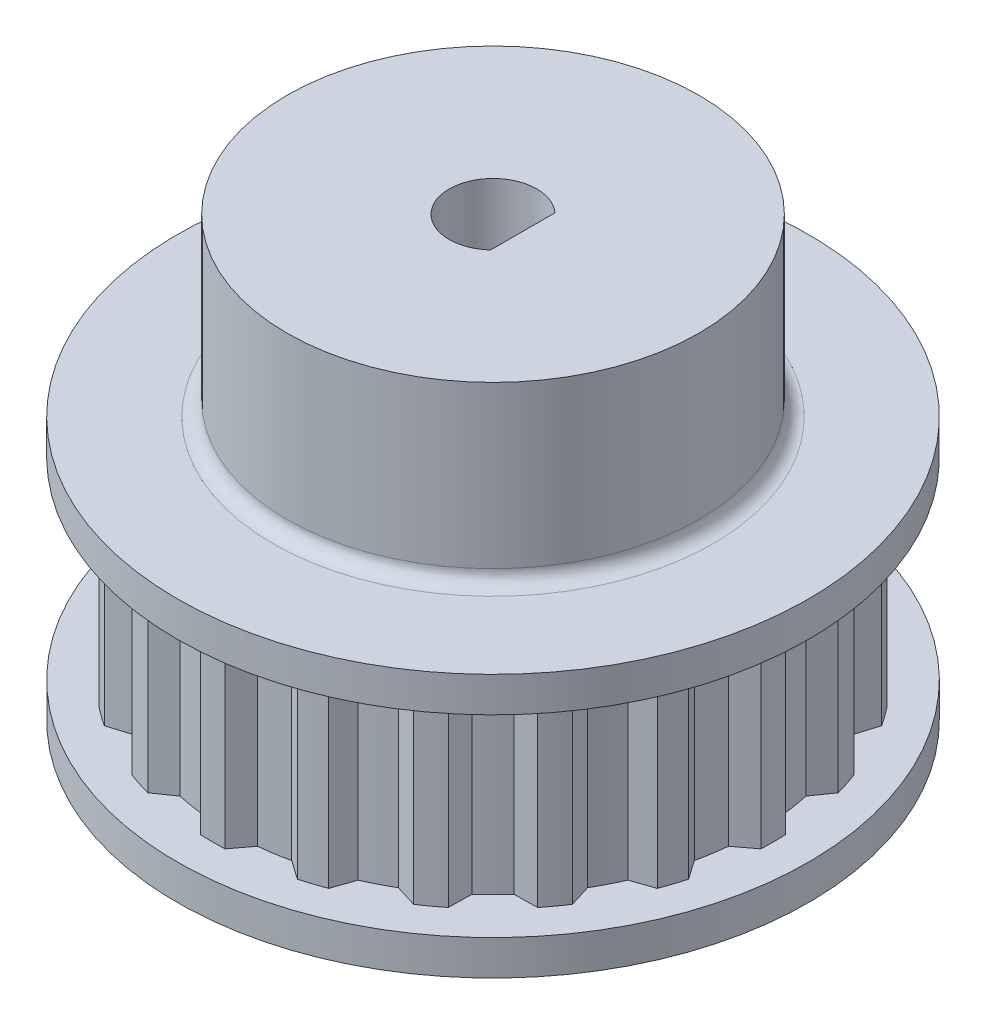
from build123d import *

# Parameters (mm, degrees)
SKETCH1_R           = 16
BOSS_EXTRUDE1_DEPTH = 11
CUT_EXTRUDE2_START  = -21
CUT_EXTRUDE2_DEPTH  = 21
SKETCH3_R           = 18
BOSS_EXTRUDE2_DEPTH = 2
BOSS_EXTRUDE3_START = 2
SKETCH4_R           = 18
BOSS_EXTRUDE3_DEPTH = 2
SKETCH5_R           = 11.75
BOSS_EXTRUDE4_DEPTH = 10
FILLET1_R           = 0.8
CUT_EXTRUDE3_DEPTH  = 52


with BuildPart() as part:
    # Sketch1 → Boss-Extrude1 (new body)
    with BuildSketch(Plane(origin=(0, 0, 0), x_dir=(1, 0, 0), z_dir=(0, 1, 0))):
        with Locations(Location((0, 0, 0), (0, 0, 270))):
            Circle(SKETCH1_R)
    extrude(amount=BOSS_EXTRUDE1_DEPTH)

    # Sketch2 → Cut-Extrude2 (cut)
    with BuildSketch(Plane(origin=(0, 11, 0), x_dir=(1, 0, 0), z_dir=(0, 1, 0)).offset(CUT_EXTRUDE2_START)):
        with BuildLine():
            ThreePointArc((4.265167024, 15.421035966), (2.502951441, 15.80301345), (0.708947293, 15.984285838))
            Line((0.708947293, 15.984285838), (1.5, 14.932939883))
            ThreePointArc((1.5, 14.932939883), (2.347782156, 14.823313142), (3.187947426, 14.665595275))
            Line((3.187947426, 14.665595275), (4.265167024, 15.421035966))
        make_face()
        with BuildLine():
            ThreePointArc((8.821777076, 13.348267649), (7.263847996, 14.256104387), (5.613664909, 14.982882443))
            Line((5.613664909, 14.982882443), (6.041116974, 13.738544292))
            ThreePointArc((6.041116974, 13.738544292), (6.813529192, 13.372303972), (7.563836345, 12.96268002))
            Line((7.563836345, 12.96268002), (8.821777076, 13.348267649))
        make_face()
        with BuildLine():
            ThreePointArc((12.514850122, 9.968877892), (11.313708499, 11.313708499), (9.968877892, 12.514850122))
            Line((9.968877892, 12.514850122), (9.990887328, 11.199324263))
            ThreePointArc((9.990887328, 11.199324263), (10.612320518, 10.612320518), (11.199324263, 9.990887328))
            Line((11.199324263, 9.990887328), (12.514850122, 9.968877892))
        make_face()
        with BuildLine():
            ThreePointArc((14.982882443, 5.613664909), (14.256104387, 7.263847996), (13.348267649, 8.821777076))
            Line((13.348267649, 8.821777076), (12.96268002, 7.563836345))
            ThreePointArc((12.96268002, 7.563836345), (13.372303972, 6.813529192), (13.738544292, 6.041116974))
            Line((13.738544292, 6.041116974), (14.982882443, 5.613664909))
        make_face()
        with BuildLine():
            ThreePointArc((15.984285838, 0.708947293), (15.80301345, 2.502951441), (15.421035966, 4.265167024))
            Line((15.421035966, 4.265167024), (14.665595275, 3.187947426))
            ThreePointArc((14.665595275, 3.187947426), (14.823313142, 2.347782156), (14.932939883, 1.5))
            Line((14.932939883, 1.5), (15.984285838, 0.708947293))
        make_face()
        with BuildLine():
            ThreePointArc((15.421035966, -4.265167024), (15.80301345, -2.502951441), (15.984285838, -0.708947293))
            Line((15.984285838, -0.708947293), (14.932939883, -1.5))
            ThreePointArc((14.932939883, -1.5), (14.823313142, -2.347782156), (14.665595275, -3.187947426))
            Line((14.665595275, -3.187947426), (15.421035966, -4.265167024))
        make_face()
        with BuildLine():
            ThreePointArc((13.348267649, -8.821777076), (14.256104387, -7.263847996), (14.982882443, -5.613664909))
            Line((14.982882443, -5.613664909), (13.738544292, -6.041116974))
            ThreePointArc((13.738544292, -6.041116974), (13.372303972, -6.813529192), (12.96268002, -7.563836345))
            Line((12.96268002, -7.563836345), (13.348267649, -8.821777076))
        make_face()
        with BuildLine():
            ThreePointArc((9.968877892, -12.514850122), (11.313708499, -11.313708499), (12.514850122, -9.968877892))
            Line((12.514850122, -9.968877892), (11.199324263, -9.990887328))
            ThreePointArc((11.199324263, -9.990887328), (10.612320518, -10.612320518), (9.990887328, -11.199324263))
            Line((9.990887328, -11.199324263), (9.968877892, -12.514850122))
        make_face()
        with BuildLine():
            ThreePointArc((5.613664909, -14.982882443), (7.263847996, -14.256104387), (8.821777076, -13.348267649))
            Line((8.821777076, -13.348267649), (7.563836345, -12.96268002))
            ThreePointArc((7.563836345, -12.96268002), (6.813529192, -13.372303972), (6.041116974, -13.738544292))
            Line((6.041116974, -13.738544292), (5.613664909, -14.982882443))
        make_face()
        with BuildLine():
            Line((1.5, -14.932939883), (0.708947293, -15.984285838))
            ThreePointArc((0.708947293, -15.984285838), (2.502951441, -15.80301345), (4.265167024, -15.421035966))
            Line((4.265167024, -15.421035966), (3.187947426, -14.665595275))
            ThreePointArc((3.187947426, -14.665595275), (2.347782156, -14.823313142), (1.5, -14.932939883))
        make_face()
        with BuildLine():
            Line((-3.187947426, -14.665595275), (-4.265167024, -15.421035966))
            ThreePointArc((-4.265167024, -15.421035966), (-2.502951441, -15.80301345), (-0.708947293, -15.984285838))
            Line((-0.708947293, -15.984285838), (-1.5, -14.932939883))
            ThreePointArc((-1.5, -14.932939883), (-2.347782156, -14.823313142), (-3.187947426, -14.665595275))
        make_face()
        with BuildLine():
            Line((-7.563836345, -12.96268002), (-8.821777076, -13.348267649))
            ThreePointArc((-8.821777076, -13.348267649), (-7.263847996, -14.256104387), (-5.613664909, -14.982882443))
            Line((-5.613664909, -14.982882443), (-6.041116974, -13.738544292))
            ThreePointArc((-6.041116974, -13.738544292), (-6.813529192, -13.372303972), (-7.563836345, -12.96268002))
        make_face()
        with BuildLine():
            Line((-11.199324263, -9.990887328), (-12.514850122, -9.968877892))
            ThreePointArc((-12.514850122, -9.968877892), (-11.313708499, -11.313708499), (-9.968877892, -12.514850122))
            Line((-9.968877892, -12.514850122), (-9.990887328, -11.199324263))
            ThreePointArc((-9.990887328, -11.199324263), (-10.612320518, -10.612320518), (-11.199324263, -9.990887328))
        make_face()
        with BuildLine():
            Line((-13.738544292, -6.041116974), (-14.982882443, -5.613664909))
            ThreePointArc((-14.982882443, -5.613664909), (-14.256104387, -7.263847996), (-13.348267649, -8.821777076))
            Line((-13.348267649, -8.821777076), (-12.96268002, -7.563836345))
            ThreePointArc((-12.96268002, -7.563836345), (-13.372303972, -6.813529192), (-13.738544292, -6.041116974))
        make_face()
        with BuildLine():
            Line((-14.932939883, -1.5), (-15.984285838, -0.708947293))
            ThreePointArc((-15.984285838, -0.708947293), (-15.80301345, -2.502951441), (-15.421035966, -4.265167024))
            Line((-15.421035966, -4.265167024), (-14.665595275, -3.187947426))
            ThreePointArc((-14.665595275, -3.187947426), (-14.823313142, -2.347782156), (-14.932939883, -1.5))
        make_face()
        with BuildLine():
            Line((-14.665595275, 3.187947426), (-15.421035966, 4.265167024))
            ThreePointArc((-15.421035966, 4.265167024), (-15.80301345, 2.502951441), (-15.984285838, 0.708947293))
            Line((-15.984285838, 0.708947293), (-14.932939883, 1.5))
            ThreePointArc((-14.932939883, 1.5), (-14.823313142, 2.347782156), (-14.665595275, 3.187947426))
        make_face()
        with BuildLine():
            Line((-12.96268002, 7.563836345), (-13.348267649, 8.821777076))
            ThreePointArc((-13.348267649, 8.821777076), (-14.256104387, 7.263847996), (-14.982882443, 5.613664909))
            Line((-14.982882443, 5.613664909), (-13.738544292, 6.041116974))
            ThreePointArc((-13.738544292, 6.041116974), (-13.372303972, 6.813529192), (-12.96268002, 7.563836345))
        make_face()
        with BuildLine():
            Line((-9.990887328, 11.199324263), (-9.968877892, 12.514850122))
            ThreePointArc((-9.968877892, 12.514850122), (-11.313708499, 11.313708499), (-12.514850122, 9.968877892))
            Line((-12.514850122, 9.968877892), (-11.199324263, 9.990887328))
            ThreePointArc((-11.199324263, 9.990887328), (-10.612320518, 10.612320518), (-9.990887328, 11.199324263))
        make_face()
        with BuildLine():
            Line((-6.041116974, 13.738544292), (-5.613664909, 14.982882443))
            ThreePointArc((-5.613664909, 14.982882443), (-7.263847996, 14.256104387), (-8.821777076, 13.348267649))
            Line((-8.821777076, 13.348267649), (-7.563836345, 12.96268002))
            ThreePointArc((-7.563836345, 12.96268002), (-6.813529192, 13.372303972), (-6.041116974, 13.738544292))
        make_face()
        with BuildLine():
            ThreePointArc((-3.187947426, 14.665595275), (-2.347782156, 14.823313142), (-1.5, 14.932939883))
            Line((-1.5, 14.932939883), (-0.708947293, 15.984285838))
            ThreePointArc((-0.708947293, 15.984285838), (-2.502951441, 15.80301345), (-4.265167024, 15.421035966))
            Line((-4.265167024, 15.421035966), (-3.187947426, 14.665595275))
        make_face()
    extrude(amount=CUT_EXTRUDE2_DEPTH, mode=Mode.SUBTRACT)

    # Sketch3 → Boss-Extrude2 (add)
    with BuildSketch(Plane(origin=(0, 11, 0), x_dir=(1, 0, 0), z_dir=(0, 1, 0))):
        with Locations(Location((0, 0, 0), (0, 0, 270))):
            Circle(SKETCH3_R)
    extrude(amount=BOSS_EXTRUDE2_DEPTH)

    # Sketch4 → Boss-Extrude3 (add)
    with BuildSketch(Plane.XZ.offset(BOSS_EXTRUDE3_START)):
        with Locations(Location((0, 0, 0), (0, 0, 90))):
            Circle(SKETCH4_R)
    extrude(amount=-BOSS_EXTRUDE3_DEPTH)

    # Sketch5 → Boss-Extrude4 (add)
    with BuildSketch(Plane(origin=(0, 13, 0), x_dir=(1, 0, 0), z_dir=(0, 1, 0))):
        with Locations(Location((0, 0, 0), (0, 0, 270))):
            Circle(SKETCH5_R)
    extrude(amount=BOSS_EXTRUDE4_DEPTH)

    # Fillet1
    fillet1_edges = [part.edges().sort_by_distance(p)[0] for p in [
        (0, 13, -11.75),
    ]]
    fillet(fillet1_edges, radius=FILLET1_R)

    # Sketch6 → Cut-Extrude3 (cut)
    with BuildSketch(Plane(origin=(0, 23, 0), x_dir=(1, 0, 0), z_dir=(0, 1, 0))):
        with BuildLine():
            Line((1.69787367, -1.835), (1.69787367, 1.835))
            ThreePointArc((1.69787367, 1.835), (-2.5, 0), (1.69787367, -1.835))
        make_face()
    extrude(amount=-CUT_EXTRUDE3_DEPTH, mode=Mode.SUBTRACT)


solid = part.part
